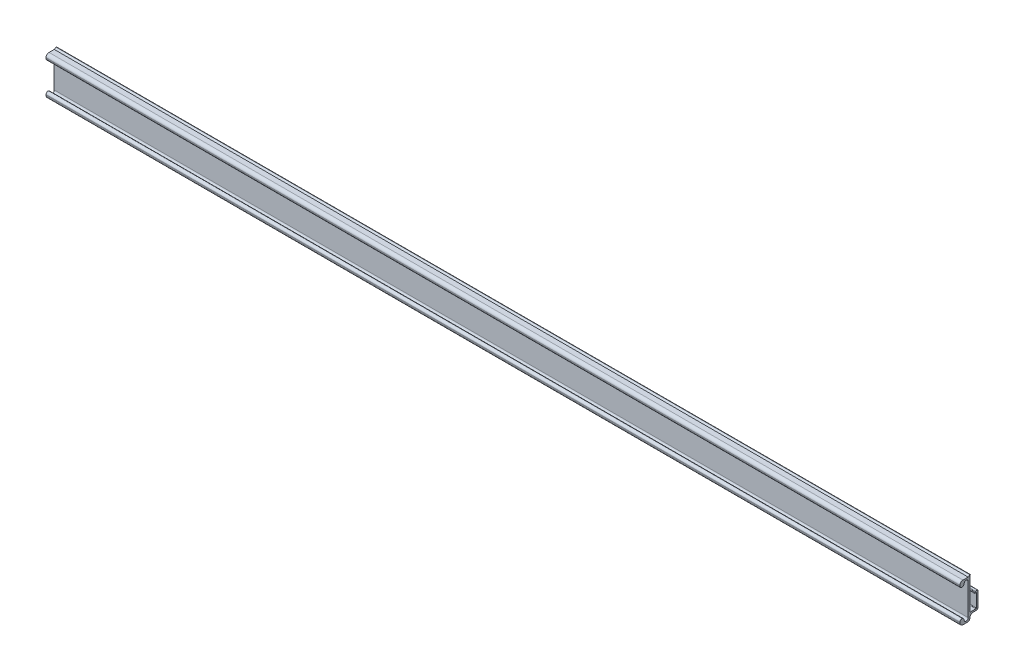
from build123d import *

# Parameters (mm, degrees)
BOSS_EXTRUDE1_DEPTH = 455


with BuildPart() as part:
    # Sketch1 → Boss-Extrude1 (new body)
    with BuildSketch(Plane(origin=(-423.5, 0, 0), x_dir=(0, -1, 0), z_dir=(-1, 0, 0))):
        with BuildLine():
            Line((-955, 454.95), (-955, 452.15))
            ThreePointArc((-955, 452.15), (-955.073223305, 451.973223305), (-955.25, 451.9))
            Line((-955.25, 451.9), (-961.9, 451.9))
            Line((-961.9, 451.9), (-961.9, 452.7))
            Line((-961.9, 452.7), (-962.45, 452.7))
            ThreePointArc((-962.45, 452.7), (-962.626776695, 452.626776695), (-962.7, 452.45))
            Line((-962.7, 452.45), (-962.7, 451.35))
            ThreePointArc((-962.7, 451.35), (-962.626776695, 451.173223305), (-962.45, 451.1))
            Line((-962.45, 451.1), (-955.2, 451.1))
            ThreePointArc((-955.2, 451.1), (-954.492893219, 451.392893219), (-954.2, 452.1))
            Line((-954.2, 452.1), (-954.2, 453.373491886))
            ThreePointArc((-954.2, 453.373491886), (-953.665028159, 454.665028159), (-952.373491886, 455.2))
            Line((-952.373491886, 455.2), (-952.3, 455.2))
            ThreePointArc((-952.3, 455.2), (-951.592893219, 455.492893219), (-951.3, 456.2))
            Line((-951.3, 456.2), (-951.3, 458.6))
            ThreePointArc((-951.3, 458.6), (-951.739339828, 459.660660172), (-952.8, 460.1))
            Line((-952.8, 460.1), (-953.2, 460.1))
            ThreePointArc((-953.2, 460.1), (-954.191183271, 459.232498012), (-953.462659626, 458.135111446))
            Line((-953.462659626, 458.135111446), (-952.837340374, 457.964888554))
            ThreePointArc((-952.837340374, 457.964888554), (-952.108816729, 456.867501988), (-953.1, 456))
            Line((-953.1, 456), (-968.799810447, 456))
            ThreePointArc((-968.799810447, 456), (-969.790988627, 456.867463908), (-969.062544211, 457.964868369))
            Line((-969.062544211, 457.964868369), (-968.437266236, 458.135131631))
            ThreePointArc((-968.437266236, 458.135131631), (-967.70882182, 459.232536092), (-968.7, 460.1))
            Line((-968.7, 460.1), (-969.1, 460.1))
            ThreePointArc((-969.1, 460.1), (-970.160660172, 459.660660172), (-970.6, 458.6))
            Line((-970.6, 458.6), (-970.6, 456))
            ThreePointArc((-970.6, 456), (-970.849658895, 455.534896264), (-971.243431907, 455.183337075))
            ThreePointArc((-971.243431907, 455.183337075), (-971.28533621, 455.130932577), (-971.284682745, 455.06383731))
            ThreePointArc((-971.284682745, 455.06383731), (-971.207838721, 454.956126495), (-971.086783129, 454.902720811))
            ThreePointArc((-971.086783129, 454.902720811), (-971.055207963, 454.903064362), (-971.025314114, 454.913236231))
            ThreePointArc((-971.025314114, 454.913236231), (-970.431156786, 455.135665686), (-969.8, 455.2))
            Line((-969.8, 455.2), (-955.25, 455.2))
            ThreePointArc((-955.25, 455.2), (-955.073223305, 455.126776695), (-955, 454.95))
        make_face()
    extrude(amount=-BOSS_EXTRUDE1_DEPTH)


solid = part.part
